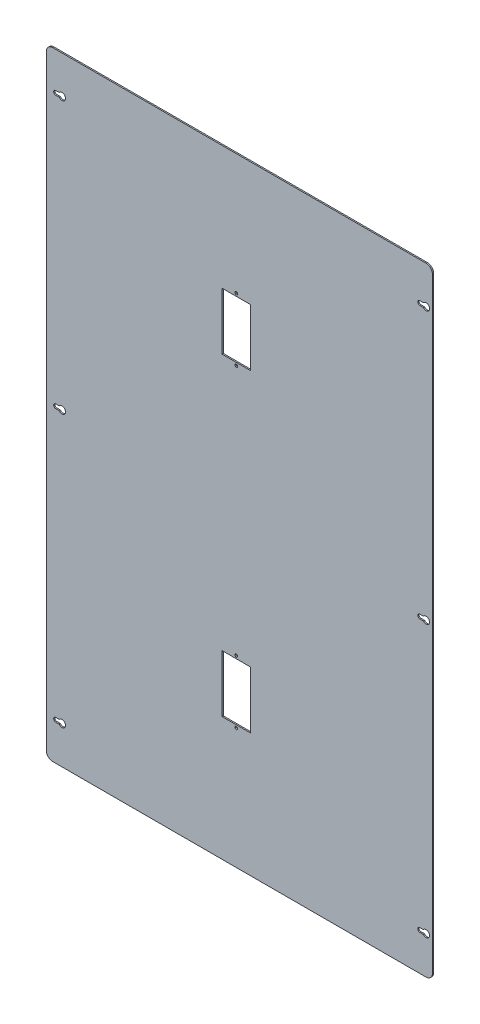
from build123d import *

# Parameters (mm, degrees)
SKETCH1_W            = 615
SKETCH1_H            = 985
BOSS_EXTRUDE1_DEPTH  = 2
SKETCH7_W            = 45
SKETCH7_H            = 91
CUT_EXTRUDE4_DEPTH   = 581.617343868
SKETCH8_R            = 2.25
CUT_EXTRUDE5_DEPTH   = 581.617343868
FILLET3_R            = 10
CUT_EXTRUDE6_DEPTH   = 10
LPATTERN1_COUNT      = 3
LPATTERN1_PITCH      = 432.5
LPATTERN1_COUNT_DIR2 = 2
LPATTERN1_PITCH_DIR2 = 580


with BuildPart() as part:
    # Sketch1 → Boss-Extrude1 (new body)
    with BuildSketch(Plane.XY):
        Rectangle(SKETCH1_W, SKETCH1_H)
    extrude(amount=BOSS_EXTRUDE1_DEPTH)

    # Sketch7 → Cut-Extrude4 (cut, through all)
    with BuildSketch(Plane(origin=(0, 0, 0), x_dir=(-1, 0, 0), z_dir=(0, 0, -1))):
        with Locations((5, 250)):
            Rectangle(SKETCH7_W, SKETCH7_H)
        with Locations((5, -250)):
            Rectangle(SKETCH7_W, SKETCH7_H)
    extrude(amount=-CUT_EXTRUDE4_DEPTH, mode=Mode.SUBTRACT)

    # Sketch8 → Cut-Extrude5 (cut, through all)
    with BuildSketch(Plane(origin=(0, 0, 0), x_dir=(-1, 0, 0), z_dir=(0, 0, -1))):
        with Locations((5, 300)):
            Circle(SKETCH8_R)
        with Locations((5, 200)):
            Circle(SKETCH8_R)
        with Locations((5, -200)):
            Circle(SKETCH8_R)
        with Locations((5, -300)):
            Circle(SKETCH8_R)
    extrude(amount=-CUT_EXTRUDE5_DEPTH, mode=Mode.SUBTRACT)

    # Fillet3
    fillet3_edges = [part.edges().sort_by_distance(p)[0] for p in [
        (307.5, -492.5, 1),
        (-307.5, -492.5, 1),
        (-307.5, 492.5, 1),
        (307.5, 492.5, 1),
    ]]
    fillet(fillet3_edges, radius=FILLET3_R)

    # Sketch10 → Cut-Extrude6 (cut)
    with BuildSketch(Plane(origin=(0, 0, 0), x_dir=(-1, 0, 0), z_dir=(0, 0, -1))):
        with BuildLine():
            Line((292.5, 435.8), (286.9, 435.8))
            ThreePointArc((286.9, 435.8), (277, 432.5), (286.9, 429.2))
            Line((286.9, 429.2), (292.5, 429.2))
            ThreePointArc((292.5, 429.2), (295.8, 432.5), (292.5, 435.8))
        make_face()
    cut_extrude6 = extrude(amount=-CUT_EXTRUDE6_DEPTH, mode=Mode.SUBTRACT)

    # LPattern1: Cut-Extrude6 3 × 2
    with Locations(*[(j * LPATTERN1_PITCH_DIR2, -i * LPATTERN1_PITCH, 0) for i in range(LPATTERN1_COUNT) for j in range(LPATTERN1_COUNT_DIR2) if (i, j) != (0, 0)]):
        add(cut_extrude6, mode=Mode.SUBTRACT)


solid = part.part
